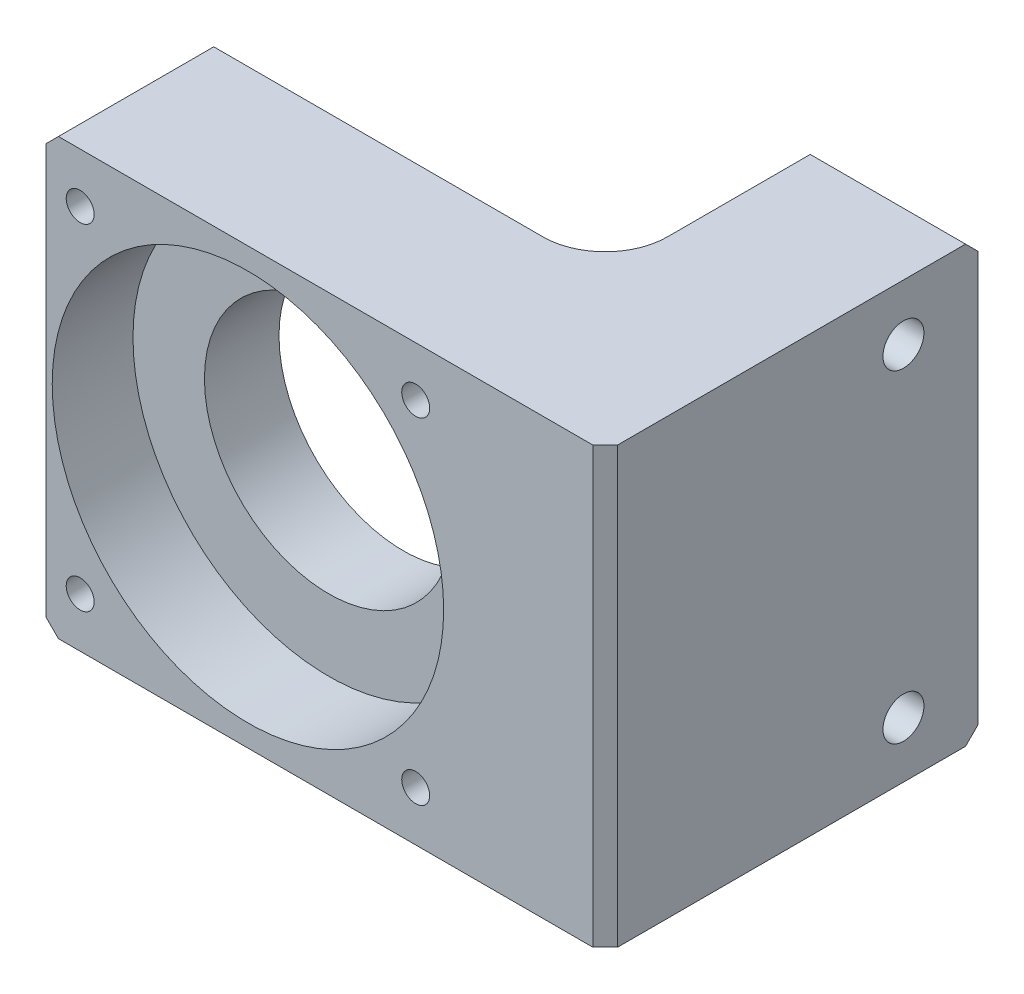
from build123d import *

# Parameters (mm, degrees)
EXTRUDE_1_DEPTH              = 35
FILLET_1_R                   = 10
SKETCH_2_R                   = 31.5
CUT_EXTRUDE_1_DEPTH          = 13
CUT_EXTRUDE_2_DEPTH          = 103.713192921
CUT_EXTRUDE_2_DEPTH_BACK     = 103.713192921
SKETCH_3_R                   = 20
HOLE_WIZARD_M6_1_D           = 6.6
HOLE_WIZARD_M6_1_CBORE_D     = 11
HOLE_WIZARD_M6_1_CBORE_DEPTH = 6.8
CHAMFER_1_SIZE               = 2
HOLE_WIZARD_M4_1_D           = 4.5
HOLE_WIZARD_M4_1_CBORE_D     = 8
HOLE_WIZARD_M4_1_CBORE_DEPTH = 43.6


with BuildPart() as part:
    # 草图1 → 凸台-拉伸1 (new, symmetric)
    with BuildSketch(Plane(origin=(0, 0, 0), x_dir=(1, 0, 0), z_dir=(0, 1, 0))):
        Polygon((0, 0), (90, 0), (90, 60), (65, 60), (65, 25), (0, 25), align=None)
    extrude(amount=EXTRUDE_1_DEPTH, both=True)

    # 圆角1
    fillet_1_edges = [part.edges().sort_by_distance(p)[0] for p in [
        (65, 0, -25),
    ]]
    fillet(fillet_1_edges, radius=FILLET_1_R)

    # 草图2 → 切除-拉伸1 (cut)
    with BuildSketch(Plane.XY):
        with Locations((32.5, 0)):
            Circle(SKETCH_2_R)
    extrude(amount=-CUT_EXTRUDE_1_DEPTH, mode=Mode.SUBTRACT)

    # 草图3 → 切除-拉伸2 (cut, two sides: drawn at the far end of the back side and taken through both)
    with BuildSketch(Plane(origin=(0, 0, -25), x_dir=(-1, 0, 0), z_dir=(0, 0, -1)).offset(-CUT_EXTRUDE_2_DEPTH_BACK)):
        with Locations((-32.5, 0)):
            Circle(SKETCH_3_R)
    extrude(amount=CUT_EXTRUDE_2_DEPTH + CUT_EXTRUDE_2_DEPTH_BACK, mode=Mode.SUBTRACT)

    # M6 六角圆柱头螺钉的柱形沉头孔1 (through all)
    with Locations(Plane.ZY.offset(-65)):
        with Locations((-48, 26), (-48, -26)):
            CounterBoreHole(HOLE_WIZARD_M6_1_D / 2, HOLE_WIZARD_M6_1_CBORE_D / 2, HOLE_WIZARD_M6_1_CBORE_DEPTH)

    # 倒角1
    chamfer_1_edges = [part.edges().sort_by_distance(p)[0] for p in [
        (90, 0, 0),
        (77.5, 35, -60),
        (0, 35, -12.5),
        (77.5, -35, -60),
        (0, -35, -12.5),
    ]]
    chamfer(chamfer_1_edges, length=CHAMFER_1_SIZE)

    # M4 六角圆柱头螺钉的柱形沉头孔1 (through all)
    with Locations(Plane(origin=(0, 0, -60), x_dir=(-1, 0, 0), z_dir=(0, 0, -1))):
        with Locations((-5.5, 27), (-59.5, 27), (-59.5, -27), (-5.5, -27)):
            CounterBoreHole(HOLE_WIZARD_M4_1_D / 2, HOLE_WIZARD_M4_1_CBORE_D / 2, HOLE_WIZARD_M4_1_CBORE_DEPTH)


solid = part.part
